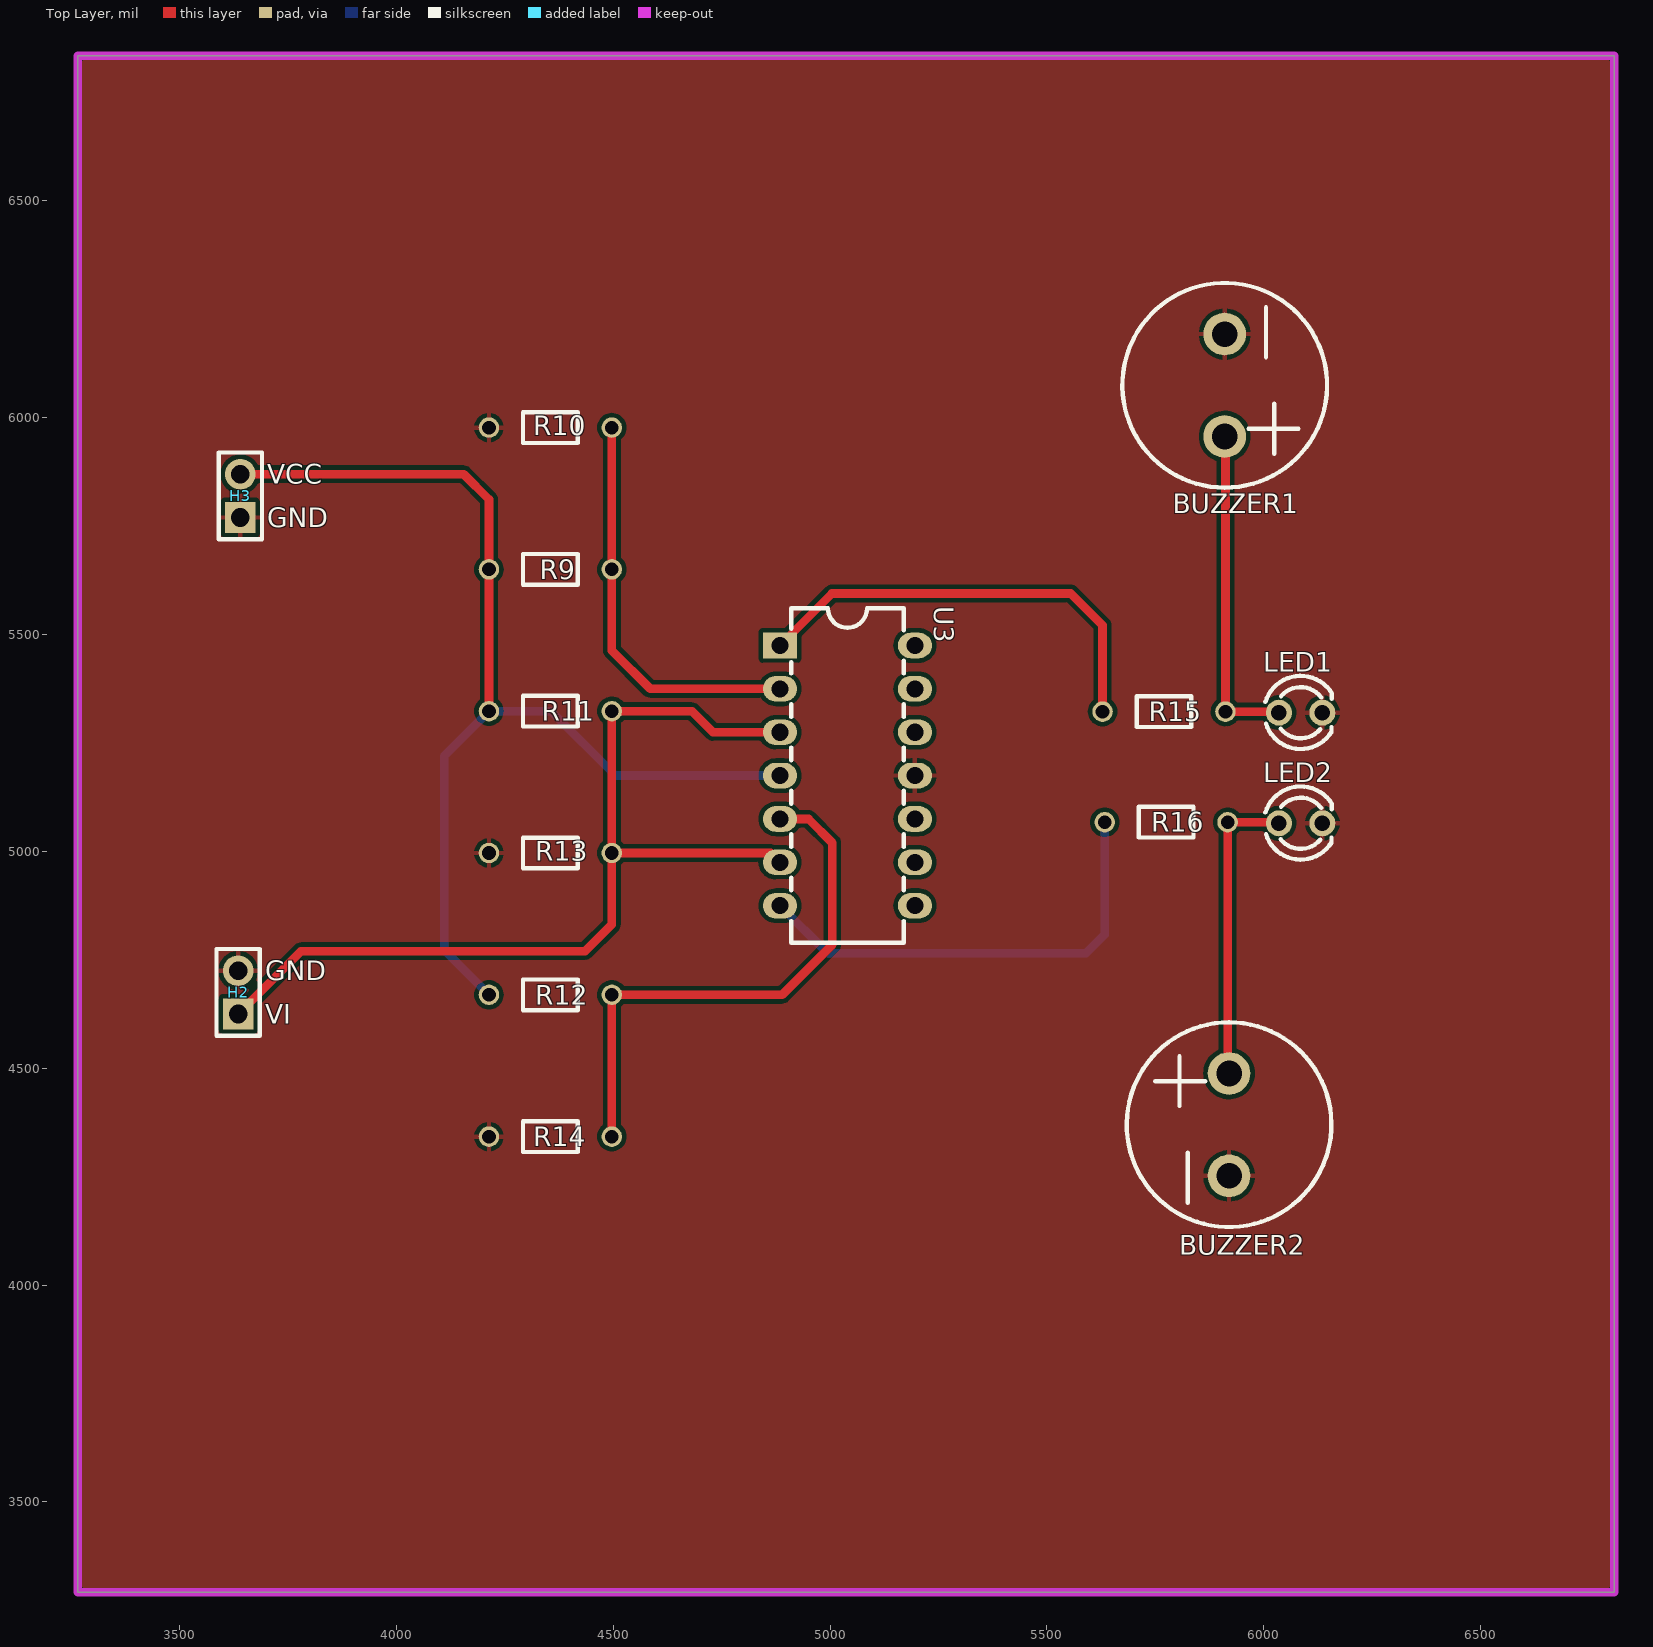
[diagram p0: Top Layer view]
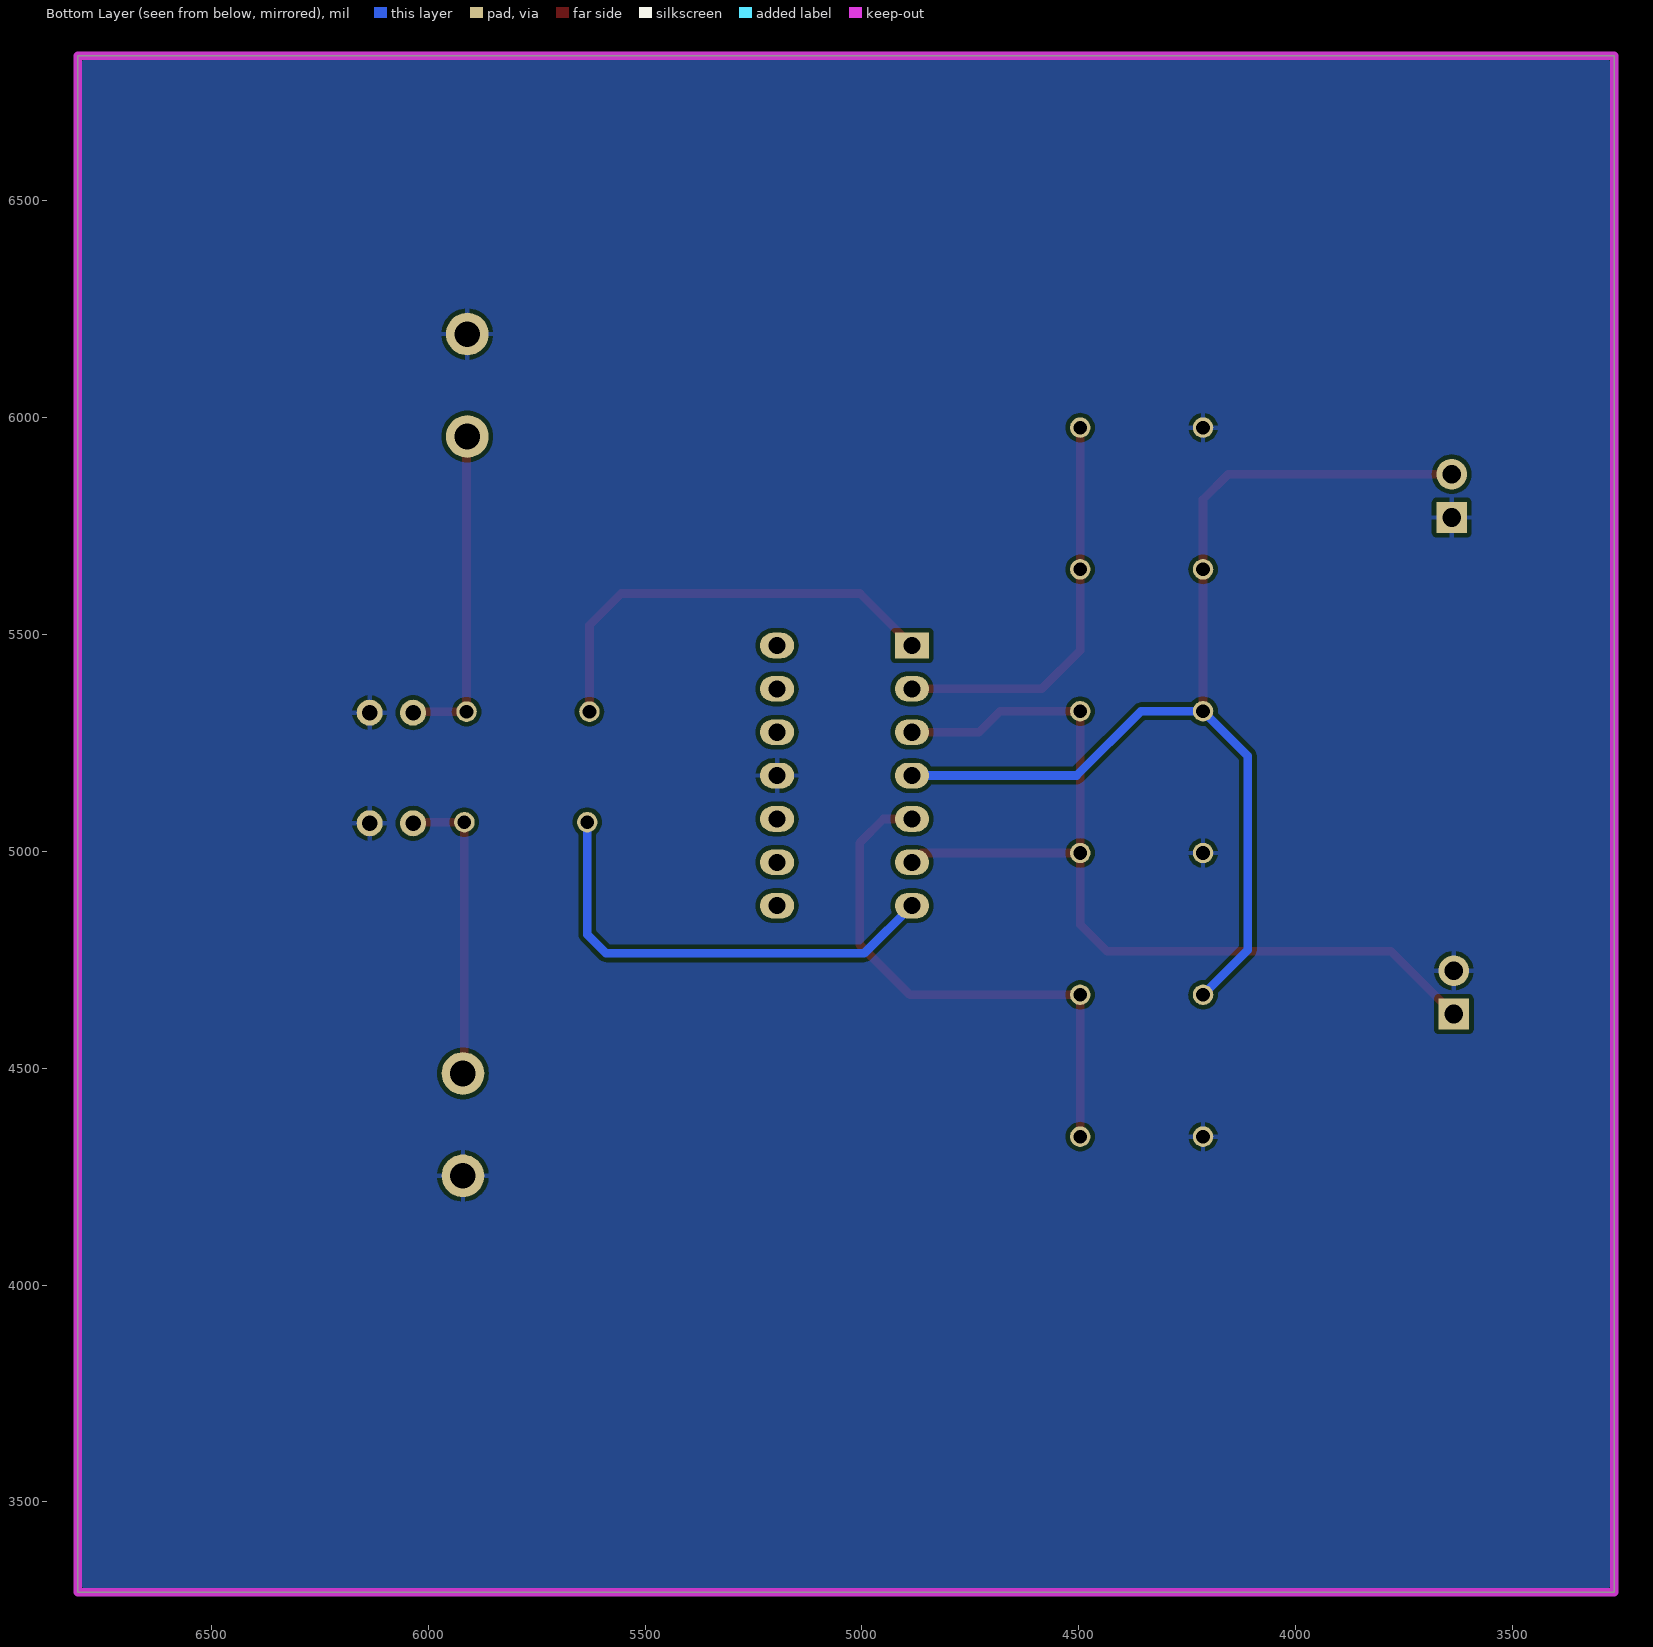
[diagram p1: Bottom Layer view, seen from below]
# Altium PCB MISC51341.pcbdoc
Units mil, origin at the board's own origin, x right, y up, seen from the top; angles counter-clockwise.
Board outline 3543.31 x 3543.31 mil, 2 copper layers (Top Layer, Bottom Layer), stack 62.206 mil thick; 15 components, 9 nets, 42 pads, 0 vias.

## Layer stack, top to bottom
Top Solder Mask Layer: solder mask 0.394, Dk 3.3
Top Layer: signal copper 1.379
Dielectric1: surface 59.449, FR4, Dk 4.5
Bottom Layer: signal copper 1.378
Bottom Solder Mask Layer: solder mask 0.394, Dk 3.3

## Board outline
3265,6835 3265,3291.69 6808.31,3291.69 6808.31,6835

## Design rules (kind name [scope] priority, off if disabled: settings)
BoardOutlineClearance copperThickness2oz_1 [All] p2 off: genericclearance=7.99 ignorepadtopadclearanceinfootprint=FALSE except(0: Arc-SplitContinuation Track-SplitContinuation SMDPad-SplitContinuation THPad-SplitContinuation Via-SplitContinuation Fill-SplitContinuation Region-SplitContinuation Poly-SplitContinuation Text-SplitContinuation Hole-SplitContinuation; 5.98: Arc-CutoutEdge Track-CutoutEdge SMDPad-CutoutEdge THPad-CutoutEdge Via-CutoutEdge Text-CutoutEdge; 6.9: Hole-OutlineEdge Hole-CutoutEdge; 10: Poly-OutlineEdge Poly-CutoutEdge; 11.81: Arc-OutlineEdge Track-OutlineEdge SMDPad-OutlineEdge THPad-OutlineEdge Via-OutlineEdge Fill-OutlineEdge Region-OutlineEdge Text-OutlineEdge Fill-CutoutEdge Region-CutoutEdge)
BoardOutlineClearance Plane_innerPlane_1 [All] p4 off: genericclearance=4.02 ignorepadtopadclearanceinfootprint=FALSE except(0: Arc-SplitContinuation Track-SplitContinuation SMDPad-SplitContinuation THPad-SplitContinuation Via-SplitContinuation Fill-SplitContinuation Region-SplitContinuation Poly-SplitContinuation Text-SplitContinuation Hole-SplitContinuation; 5.98: Arc-CutoutEdge Track-CutoutEdge SMDPad-CutoutEdge THPad-CutoutEdge Via-CutoutEdge Text-CutoutEdge; 6.9: Hole-OutlineEdge Hole-CutoutEdge; 10: Poly-OutlineEdge Poly-CutoutEdge; 11.81: Arc-OutlineEdge Track-OutlineEdge SMDPad-OutlineEdge THPad-OutlineEdge Via-OutlineEdge Fill-OutlineEdge Region-OutlineEdge Text-OutlineEdge Fill-CutoutEdge Region-CutoutEdge)
BoardOutlineClearance Copper_copperRegion_1 [All] p6 off: genericclearance=4.02 ignorepadtopadclearanceinfootprint=FALSE except(0: Arc-SplitContinuation Track-SplitContinuation SMDPad-SplitContinuation THPad-SplitContinuation Via-SplitContinuation Fill-SplitContinuation Region-SplitContinuation Poly-SplitContinuation Text-SplitContinuation Hole-SplitContinuation; 5.98: Arc-CutoutEdge Track-CutoutEdge SMDPad-CutoutEdge THPad-CutoutEdge Via-CutoutEdge Text-CutoutEdge; 6.9: Hole-OutlineEdge Hole-CutoutEdge; 10: Poly-OutlineEdge Poly-CutoutEdge; 11.81: Arc-OutlineEdge Track-OutlineEdge SMDPad-OutlineEdge THPad-OutlineEdge Via-OutlineEdge Fill-OutlineEdge Region-OutlineEdge Text-OutlineEdge Fill-CutoutEdge Region-CutoutEdge)
BoardOutlineClearance copperThickness1oz_1 [All] p8: genericclearance=4.02 ignorepadtopadclearanceinfootprint=FALSE except(0: Arc-SplitContinuation Track-SplitContinuation SMDPad-SplitContinuation THPad-SplitContinuation Via-SplitContinuation Fill-SplitContinuation Region-SplitContinuation Poly-SplitContinuation Text-SplitContinuation Hole-SplitContinuation; 5.98: Arc-CutoutEdge Track-CutoutEdge SMDPad-CutoutEdge THPad-CutoutEdge Via-CutoutEdge Text-CutoutEdge; 6.9: Hole-OutlineEdge Hole-CutoutEdge; 10: Poly-OutlineEdge Poly-CutoutEdge; 11.81: Arc-OutlineEdge Track-OutlineEdge SMDPad-OutlineEdge THPad-OutlineEdge Via-OutlineEdge Fill-OutlineEdge Region-OutlineEdge Text-OutlineEdge Fill-CutoutEdge Region-CutoutEdge)
Clearance copperThickness2oz [All] p1 off: gap=7.99 ignorepadtopadclearanceinfootprint=FALSE except(5.98: SMDPad-Track SMDPad-SMDPad THPad-Track SMDPad-THPad THPad-THPad Track-Via SMDPad-Via THPad-Via Via-Via Fill-SMDPad Region-SMDPad Fill-THPad Region-THPad Fill-Via Region-Via Fill-Fill Fill-Region Region-Region Arc-Track Arc-SMDPad Arc-THPad Arc-Via Fill-Arc Region-Arc Arc-Arc Text-Track SMDPad-Text Text-THPad Text-Via Fill-Text Region-Text Arc-Text Text-Text; 6.9: Hole-Track Hole-SMDPad Hole-THPad Hole-Via Fill-Hole Region-Hole Hole-Arc Hole-Text; 10: Poly-Track Poly-SMDPad Poly-THPad Poly-Via Poly-Fill Poly-Region Poly-Poly Poly-Arc Poly-Text Poly-Hole; 11.81: Fill-Track Region-Track)
Clearance Plane_innerPlane [All] p3 off: gap=4.02 ignorepadtopadclearanceinfootprint=FALSE except(5.98: SMDPad-Track SMDPad-SMDPad THPad-Track SMDPad-THPad THPad-THPad Track-Via SMDPad-Via THPad-Via Via-Via Fill-SMDPad Region-SMDPad Fill-THPad Region-THPad Fill-Via Region-Via Fill-Fill Fill-Region Region-Region Arc-Track Arc-SMDPad Arc-THPad Arc-Via Fill-Arc Region-Arc Arc-Arc Text-Track SMDPad-Text Text-THPad Text-Via Fill-Text Region-Text Arc-Text Text-Text; 6.9: Hole-Track Hole-SMDPad Hole-THPad Hole-Via Fill-Hole Region-Hole Hole-Arc Hole-Text; 10: Poly-Track Poly-SMDPad Poly-THPad Poly-Via Poly-Fill Poly-Region Poly-Poly Poly-Arc Poly-Text Poly-Hole; 11.81: Fill-Track Region-Track)
Clearance Copper_copperRegion [All] p5 off: gap=4.02 ignorepadtopadclearanceinfootprint=FALSE except(5.98: SMDPad-Track SMDPad-SMDPad THPad-Track SMDPad-THPad THPad-THPad Track-Via SMDPad-Via THPad-Via Via-Via Fill-SMDPad Region-SMDPad Fill-THPad Region-THPad Fill-Via Region-Via Fill-Fill Fill-Region Region-Region Arc-Track Arc-SMDPad Arc-THPad Arc-Via Fill-Arc Region-Arc Arc-Arc Text-Track SMDPad-Text Text-THPad Text-Via Fill-Text Region-Text Arc-Text Text-Text; 6.9: Hole-Track Hole-SMDPad Hole-THPad Hole-Via Fill-Hole Region-Hole Hole-Arc Hole-Text; 10: Poly-Track Poly-SMDPad Poly-THPad Poly-Via Poly-Fill Poly-Region Poly-Poly Poly-Arc Poly-Text Poly-Hole; 11.81: Fill-Track Region-Track)
Clearance copperThickness1oz [All] p7: gap=4.02 ignorepadtopadclearanceinfootprint=FALSE except(5.98: SMDPad-Track SMDPad-SMDPad THPad-Track SMDPad-THPad THPad-THPad Track-Via SMDPad-Via THPad-Via Via-Via Fill-SMDPad Region-SMDPad Fill-THPad Region-THPad Fill-Via Region-Via Fill-Fill Fill-Region Region-Region Arc-Track Arc-SMDPad Arc-THPad Arc-Via Fill-Arc Region-Arc Arc-Arc Text-Track SMDPad-Text Text-THPad Text-Via Fill-Text Region-Text Arc-Text Text-Text; 6.9: Hole-Track Hole-SMDPad Hole-THPad Hole-Via Fill-Hole Region-Hole Hole-Arc Hole-Text; 10: Poly-Track Poly-SMDPad Poly-THPad Poly-Via Poly-Fill Poly-Region Poly-Poly Poly-Arc Poly-Text Poly-Hole; 11.81: Fill-Track Region-Track)
DiffPairsRouting differentialPair [All] p1: maxlimit=6 minlimit=6 mostfreqgap=6 toplayer_minwidth=5 toplayer_prefwidth=10 toplayer_maxwidth=100 toplayer_mingap=6 toplayer_prefgap=6 toplayer_maxgap=6 bottomlayer_minwidth=5 bottomlayer_prefwidth=10 bottomlayer_maxwidth=100 bottomlayer_mingap=6 bottomlayer_prefgap=6 bottomlayer_maxgap=6 maxuncoupledlength=10
HoleToHoleClearance otherClearance [All] p1: gap=11.81 allowstackedmicrovias=TRUE
Length netLength [All] p1: minlimit=0 maxlimit=0
PasteMaskExpansion pasteMaskExpansion [All] p1: expansion=0
PlaneConnect innerPlane [All] p1: planeconnectstyle=Relief reliefexpansion=20 reliefentries=4 reliefconductorwidth=10 reliefairgap=10
PolygonConnect copperRegion [All] p1: connectstyle=Relief reliefconductorwidth=10 reliefentries=4 polygonreliefangle="90 Angle" airgapwidth=10 via.connectstyle=Relief via.reliefconductorwidth=10 via.reliefentries=4 via.polygonreliefangle="90 Angle" via.airgapwidth=10
RoutingVias viaSize [All] p1: holewidth=12.01 width=24.02 viastyle="Through Hole" minholewidth=11.81 minwidth=19.68 maxholewidth=248.03 maxwidth=393.7
SolderMaskExpansion solderMaskExpansion [IsVia] p1: expansion=-1000 istentingtop=TRUE
SolderMaskExpansion solderMaskExpansion [All] p2: expansion=2 istentingtop=FALSE
Width copperThickness2oz_2 [All] p1 off: maxlimit=100 minlimit=8 preferedwidth=10
Width copperThickness1oz_2 [All] p2: maxlimit=100 minlimit=5 preferedwidth=10

## Components (designator, comment, footprint, x,y, rotation, side; value= is the part's Value field where it differs from the comment)
BUZZER1 "buzzer" BUZ-TH_BD12.0-P6.00-D0.9-RD 5910,6075 r270 top
BUZZER2 "buzzer" BUZ-TH_BD12.0-P6.00-D0.9-RD 5920,4370 r90 top
H2 "" HDR-TH_2P-P2.54-V-M-1 3635,4675 r90 top
H3 "" HDR-TH_2P-P2.54-V-M-1 3640,5820 r90 top
LED1 "" LED_TH-3mm 6085,5320 r0 top
LED2 "" LED_TH-3mm 6085,5065 r0 top
R9 "30K" Res_1/8W 4355,5648 r0 top
R10 "68K" Res_1/8W 4355,5975 r0 top
R11 "30K" Res_1/8W 4355,5325.95 r180 top
R12 "68K" Res_1/8W 4355,4667 r0 top
R13 "51K" Res_1/8W 4355,4994 r0 top
R14 "13K" Res_1/8W 4355,4340 r0 top
R15 "220" Res_1/8W 5770,5320 r0 top
R16 "220" Res_1/8W 5775,5065 r0 top
U3 "LM324ANE4" PDIP-14_L19.6-W6.5-P2.54-LS7.9-BL 5040,5175 r270 top

## Footprints (in the part's own frame and the unit in brackets; to place one, negate y for a bottom-side part, rotate by r counter-clockwise, add the part's x,y. Pads: shape width x height; smd on the part's side, far side on the other; paste and mask are expansions set on the pad)
BUZ-TH_BD12.0-P6.00-D0.9-RD [mm]
  round 2.5 hole 1.5 paste+0 mask+0.05: 1(-3,0) 2(3,0)
  silkscreen extent -5.99,-5.99 5.99,5.99
HDR-TH_2P-P2.54-V-M-1 [mm]
  rect 1.8x1.8 hole 1.1: 1(-1.27,0)
  round 1.8 hole 1.1: 2(1.27,0)
  silkscreen extent -2.54,-1.27 2.54,1.27
LED_TH-3mm [mil]
  round 60 hole 36 paste+0 mask+2: 1(-50,0) 2(50,0)
  silkscreen extent -81,-84 72,85
PDIP-14_L19.6-W6.5-P2.54-LS7.9-BL [mm]
  rect 1.5x2 hole 1: 1(-7.62,-3.95)
  oval 1.5x2 hole 1: 2(-5.08,-3.95) 3(-2.54,-3.95) 4(0,-3.95) 5(2.54,-3.95) 6(5.08,-3.95) 7(7.62,-3.95) 8(7.62,3.95) 9(5.08,3.95) 10(2.54,3.95) 11(0,3.95) 12(-2.54,3.95) 13(-5.08,3.95) 14(-7.62,3.95)
  silkscreen extent -9.8,-3.3 9.8,3.3
Res_1/8W [mil]
  round 47.2 hole 31.5 paste+0 mask+2: 1(-141.7,2.48) 2(141.7,2.48)
  silkscreen extent -63,-33 63,38

## Nets (pads, with @x,y where several pads share a name; then routed paths per layer and width w, separated by ;. In a path a pad name is that pad's centre, name@x,y a point inside that pad or via, vN(x,y) a via of type N, cw(c..) or ccw(c..) an arc to the next point about the centre after c; other vN are vias at no path point)
$1N193: R9.2 R10.2 U3.2 | length 938.5
  Top Layer w20: R10.2 R9.2 4496.7,5463.3 4585,5375 U3.2
$1N797: R12.2 R14.2 U3.5 | length 1261.4
  Top Layer w20: R14.2 R12.2 4889.48,4669.48 5005,4785 5005,5020 4950,5075 U3.5
$1N964: BUZZER1.2 LED1.1 R15.2 | length 759.4
  Top Layer w20: BUZZER1.2 5911.7,5955.19 R15.2 6032.52,5322.48 LED1.1
$1N967: R15.1 U3.1 | length 1023.1
  Top Layer w20: U3.1 5004.49,5595 5555,5595 5628.3,5521.7 R15.1
$1N1018: BUZZER2.2 LED2.1 R16.2 | length 700.1
  Top Layer w20: BUZZER2.2 5916.7,4491.41 R16.2 6032.52,5067.48 LED2.1
$1N1021: R16.1 U3.7 | length 1071.5
  Bottom Layer w20: U3.7 4994.49,4765 5590,4765 5633.3,4808.3 R16.1
GND: BUZZER1.1 BUZZER2.1 H2.2 H3.1 LED1.2 LED2.2 R10.1 R13.1 R14.1 U3.11
VCC: H3.2 R9.1 R11.2 R12.1 U3.4 | length 2557.9
  Top Layer w20: H3.2 4155,5870 4213.3,5811.7 R9.1 R11.2
  Bottom Layer w20: R12.1 4110,4772.78 4110,5220.18 R11.2 4356.52,5323.48 4505,5175 U3.4
VI: H2.1 R11.1 R13.2 U3.3 U3.6 | length 2243.7
  Top Layer w20: H2.1 3780,4770 4435,4770 4496.7,4831.7 R13.2 ; U3.6 4863.01,4996.48 R13.2 ; U3.3 4730,5275 4681.52,5323.48 R11.1 R13.2
pads on no net: U3.8 U3.9 U3.10 U3.12 U3.13 U3.14

## Polygon pours and split planes (outlines as drawn)
GND on Top Layer (solid, remove dead copper, pour order 0): 3080,6965 3080,3225 7245,3225 7245,6965
GND on Bottom Layer (solid, remove dead copper, pour order 2): 3000,6985 3000,3000 6985,3000 6985,6985

## Keep-outs
Board Outline Layer:
  the board outline again, w20

## Silkscreen, mask and mechanical layers (free items; w line width, h text height)
Top Silkscreen Layer:
  text "VCC" at 3702.42,5847.5 h45
  text "GND" at 3702.42,5747.5 h45
  text "GND" at 3697.42,4702.5 h45
  text "VI" at 3697.42,4602.5 h45